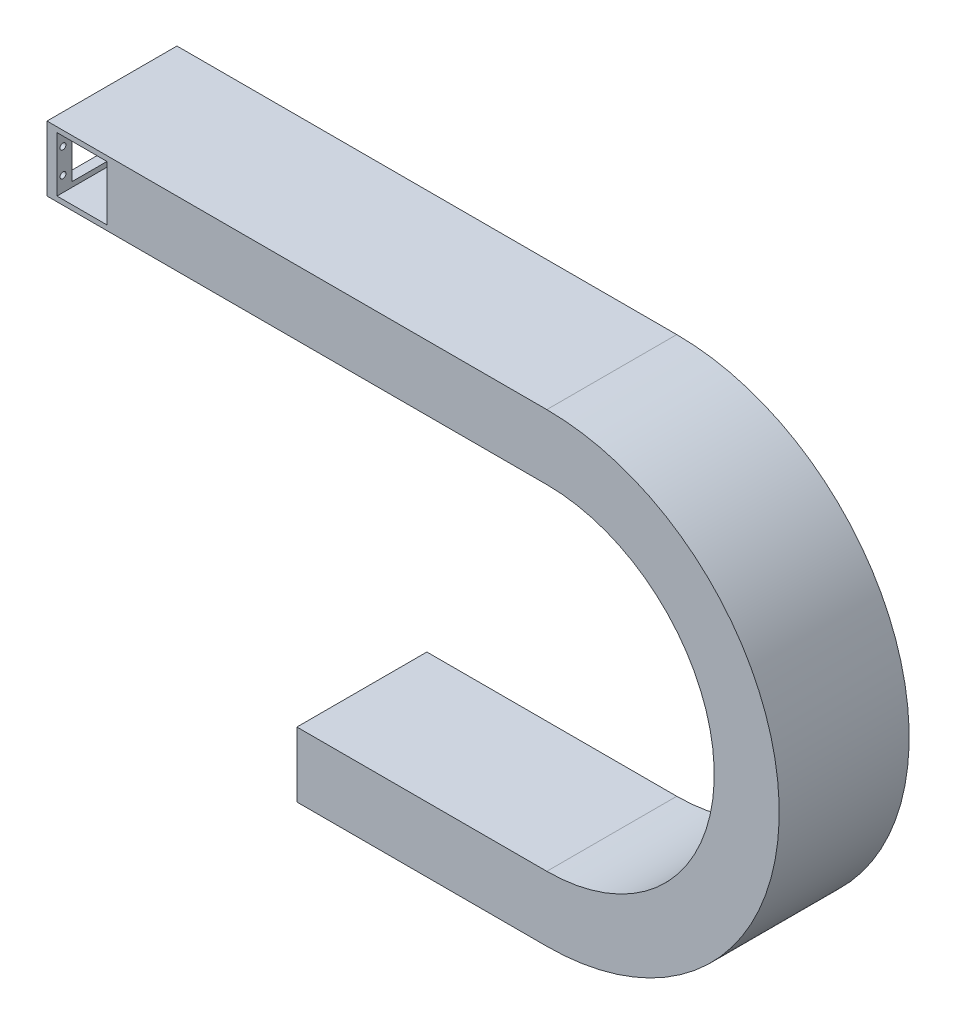
from build123d import *

# Parameters (mm, degrees)
EXTRUDE_1_DEPTH     = 130
SKETCH_2_R          = 3
CUT_EXTRUDE_1_DEPTH = 20
SKETCH_9_W          = 50
SKETCH_9_H          = 55
CUT_EXTRUDE_2_DEPTH = 150
SKETCH_10_W         = 100
SKETCH_10_H         = 45
CUT_EXTRUDE_3_DEPTH = 200


with BuildPart() as part:
    # 草图1 → 凸台-拉伸1 (new body)
    with BuildSketch(Plane.XY):
        with BuildLine():
            Line((-450.427662897, 234.022122697), (-950.427662897, 234.022122697))
            Line((-950.427662897, 234.022122697), (-950.427662897, 299.022122697))
            Line((-950.427662897, 299.022122697), (-450.427662897, 299.022122697))
            ThreePointArc((-450.427662897, 299.022122697), (-217.927662897, 66.522122697), (-450.427662897, -165.977877303))
            Line((-450.427662897, -165.977877303), (-700.427662897, -165.977877303))
            Line((-700.427662897, -165.977877303), (-700.427662897, -100.977877303))
            Line((-700.427662897, -100.977877303), (-450.427662897, -100.977877303))
            ThreePointArc((-450.427662897, -100.977877303), (-282.927662897, 66.522122697), (-450.427662897, 234.022122697))
        make_face()
    extrude(amount=EXTRUDE_1_DEPTH)

    # 草图2 → 切除-拉伸1 (cut)
    with BuildSketch(Plane.ZY.offset(950.427662897)):
        with Locations((6, 279.022122697)):
            Circle(SKETCH_2_R)
        with Locations((6, 254.022122697)):
            Circle(SKETCH_2_R)
        with Locations((124, 279.022122697)):
            Circle(SKETCH_2_R)
        with Locations((124, 254.022122697)):
            Circle(SKETCH_2_R)
    extrude(amount=-CUT_EXTRUDE_1_DEPTH, mode=Mode.SUBTRACT)

    # 草图9 → 切除-拉伸2 (cut)
    with BuildSketch(Plane.XY.offset(130)):
        with Locations((-915.427662897, 266.522122697)):
            Rectangle(SKETCH_9_W, SKETCH_9_H)
    extrude(amount=-CUT_EXTRUDE_2_DEPTH, mode=Mode.SUBTRACT)

    # 草图10 → 切除-拉伸3 (cut)
    with BuildSketch(Plane.ZY.offset(950.427662897)):
        with Locations((65, 266.522122697)):
            Rectangle(SKETCH_10_W, SKETCH_10_H)
    extrude(amount=-CUT_EXTRUDE_3_DEPTH, mode=Mode.SUBTRACT)


solid = part.part
